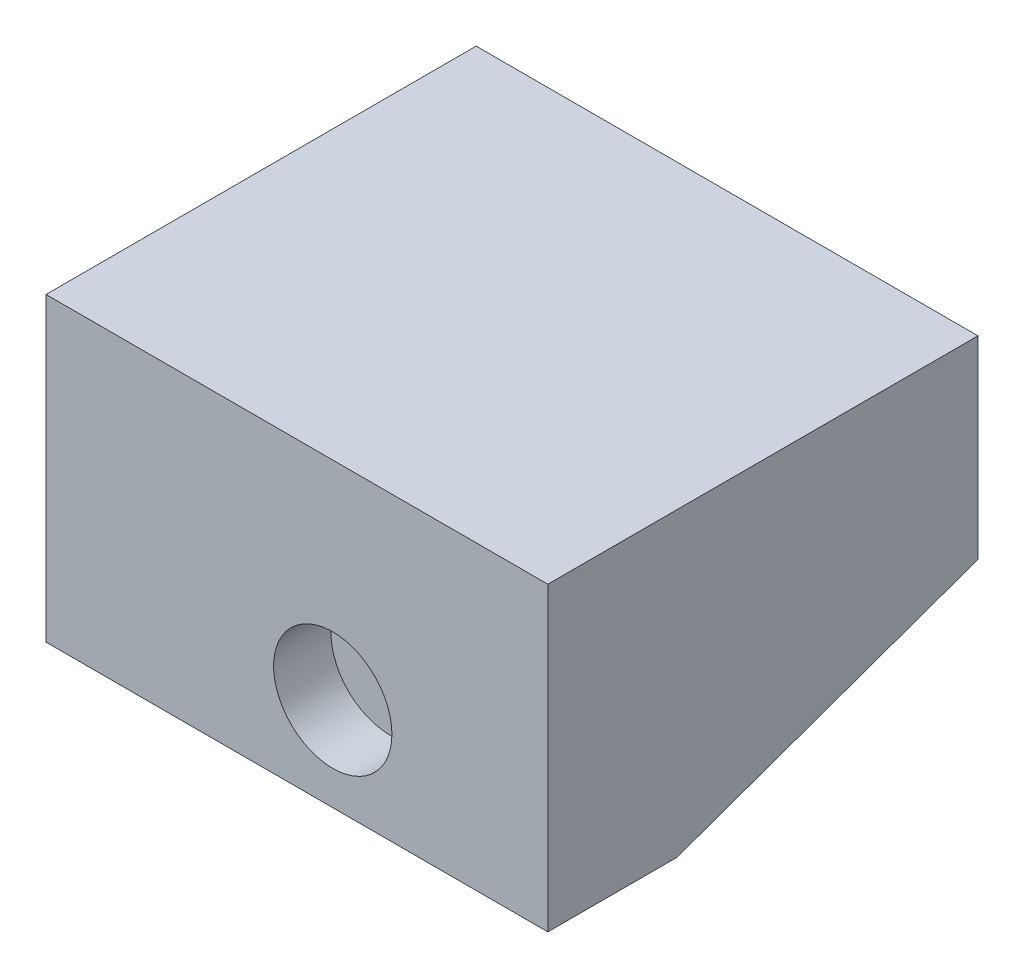
from build123d import *

# Parameters (mm, degrees)
SKETCH1_W           = 60
SKETCH1_H           = 60
BOSS_EXTRUDE1_DEPTH = 20
BOSS_EXTRUDE2_DEPTH = 70
SKETCH8_R           = 8.25
CUT_EXTRUDE5_DEPTH  = 8


with BuildPart() as part:
    # Sketch1 → Boss-Extrude1 (new body)
    with BuildSketch(Plane(origin=(0, 0, 0), x_dir=(1, 0, 0), z_dir=(0, 1, 0))):
        Rectangle(SKETCH1_W, SKETCH1_H)
    extrude(amount=BOSS_EXTRUDE1_DEPTH)

    # Sketch2 → Boss-Extrude2 (add)
    with BuildSketch(Plane(origin=(30, 0, 0), x_dir=(0, 0, -1), z_dir=(1, 0, 0))):
        Polygon((30, 20), (30, 0), (30, -7), (-12, -22), (-30, -22), (-30, 20), align=None)
    extrude(amount=-BOSS_EXTRUDE2_DEPTH)

    # Sketch8 → Cut-Extrude5 (cut)
    with BuildSketch(Plane.XY.offset(30)):
        with Locations((0, -9)):
            Circle(SKETCH8_R)
    extrude(amount=-CUT_EXTRUDE5_DEPTH, mode=Mode.SUBTRACT)


solid = part.part
